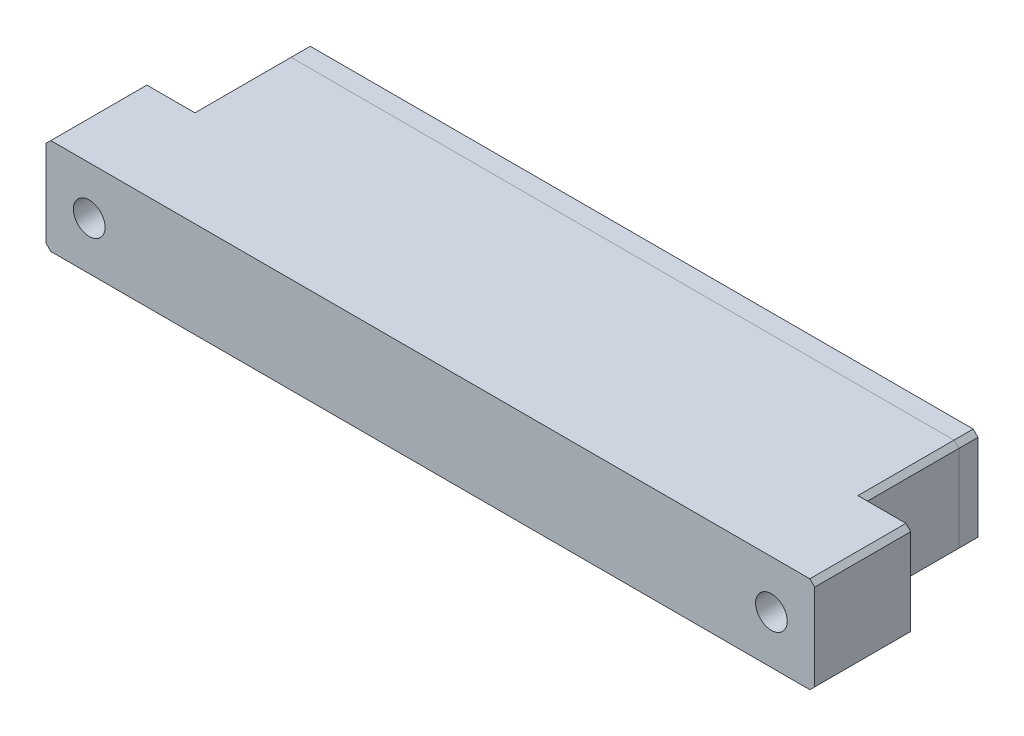
SolidWorks part; units mm, degrees
material "A6063"
ref_plane "Front Plane" through (0, 0, 0) normal (0, 0, 1) x (1, 0, 0)
ref_plane "Top Plane" through (0, 0, 0) normal (0, 1, 0) x (1, 0, 0)
ref_plane "Right Plane" through (0, 0, 0) normal (1, 0, 0) x (0, 0, -1)
sketch "Sketch1" plane through (0, 0, 0) normal (0, 0, 1) x (1, 0, 0)
  line L1 (40, -5) -> (-40, -5)
  line L2 (40, -5) -> (40, 5)
  line L3 (40, 5) -> (-40, 5)
  line L4 (-40, -5) -> (-40, 5)
  line L5 (40, -5) -> (-40, 5) construction
  line L6 (40, 5) -> (-40, -5) construction
  point P0 (0, 0)
  dimension "D1" = 80
  dimension "D2" = 10
extrude "Boss-Extrude1" add sketch "Sketch1" along normal blind 20
sketch "Sketch9" plane through (0, 5, 0) normal (0, 1, 0) x (1, 0, 0)
  line L0 (0, 0) -> (0, -36.7586) construction
  line L1 (40, 0) -> (35, 0)
  line L2 (40, 0) -> (40, -10)
  line L3 (40, -10) -> (35, -10)
  line L4 (35, 0) -> (35, -10)
  line L5 (-40, 0) -> (-35, 0)
  line L6 (-40, 0) -> (-40, -10)
  line L7 (-40, -10) -> (-35, -10)
  line L8 (-35, 0) -> (-35, -10)
  dimension "D1" = 70
  dimension "D2" = 10
extrude "Cut-Extrude3" cut sketch "Sketch9" against normal through all
hole_wizard "M4 Tapped Hole1" positions "Sketch4" profile "Sketch3" tap size "M4" standard "GB"
sketch "Sketch4" plane through (0, 0, 20) normal (0, 0, 1) x (1, 0, 0)
  line L0 (0, 7.9254) -> (0, 0) construction
  line L1 (0, 0) -> (18.9615, 0) construction
  point P0 (-35.5, 0)
  point P1 (35.5, 0)
  dimension "D1" = 71
sketch "Sketch3" plane through (-35.5, 0, 20) normal (1, 0, 0) x (0, -1, 0)
  line L0 (0, 0) -> (0, 8.9914)
  line L1 (0, 8.9914) -> (1.65, 8)
  line L2 (1.65, 8) -> (1.65, 0)
  line L5 (1.65, 0) -> (0, 0)
  line L10 (0, 8.9914) -> (-1.65, 8) construction
  line L11 (0, -6.35) -> (0, 107.95) construction
  dimension "螺纹孔钻头直径" = 3.3
  dimension "螺纹孔钻头深度" = 8
  dimension "导头角度" = 118
cosmetic thread "Cosmetic Thread3" parameters "D1"=8, "D2"=4
cosmetic thread "Cosmetic Thread4" parameters "D1"=8, "D2"=4
hole_wizard "M5 Tapped Hole1" positions "Sketch7" profile "Sketch6" tap size "M5" standard "GB"
sketch "Sketch7" plane through (0, -5, 0) normal (0, -1, 0) x (1, 0, 0)
  line L1 (0, 0) -> (0, 6.5) construction
  line L2 (-35, 0) -> (35, 0) construction
  point P0 (0, 6.5)
  dimension "D1" = 6.5
sketch "Sketch6" plane through (0, -5, 6.5) normal (1, 0, 0) x (0, 0, -1)
  line L0 (0, 0) -> (0, 8)
  line L1 (0, 8) -> (2.1, 8)
  line L2 (2.1, 8) -> (2.1, 0)
  line L5 (2.1, 0) -> (0, 0)
  line L10 (0, 8) -> (-2.1, 8) construction
  line L11 (0, -6.35) -> (0, 107.95) construction
  dimension "螺纹孔钻头直径" = 4.2
  dimension "螺纹孔钻头深度" = 8
  dimension "导头角度" = 180
cosmetic thread "Cosmetic Thread5" parameters "D1"=2, "D2"=5
sketch "Sketch8" plane through (0, 0, 0) normal (0, 0, -1) x (-1, 0, 0)
  line L0 (0, 0) -> (25.8164, 0) construction
  line L2 (-34, 4) -> (34, 4)
  line L3 (-34, 4) -> (-34, -4)
  line L4 (-34, -4) -> (34, -4)
  line L7 (34, 4) -> (34, -4)
  line L8 (0, 0) -> (0, -13.1501) construction
  line L9 (-35, 5) -> (35, 5) construction
  line L10 (35, -5) -> (35, 5) construction
  dimension "D1" = 1
  dimension "D2" = 1
extrude "Cut-Extrude2" cut sketch "Sketch8" against normal blind 3
sketch "Sketch10" plane through (0, 0, 3) normal (0, 0, -1) x (-1, 0, 0)
  line L0 (0, 0) -> (18.7293, 0) construction
  line L1 (-32, 3) -> (32, 3)
  line L2 (-32, 3) -> (-32, -3)
  line L3 (-32, -3) -> (32, -3)
  line L4 (32, 3) -> (32, -3)
  line L5 (0, 0) -> (0, 14.5079) construction
  line L6 (34, 4) -> (-34, 4) construction
  line L7 (34, -4) -> (34, 4) construction
  dimension "D1" = 1
  dimension "D2" = 2
extrude "Cut-Extrude4" cut sketch "Sketch10" against normal blind 3.5
sketch "Sketch11" plane through (0, 0, 3) normal (0, 0, -1) x (-1, 0, 0)
  line L1 (-34, 4) -> (34, 4)
  line L2 (-34, 4) -> (-34, -4)
  line L3 (-34, -4) -> (34, -4)
  line L4 (34, 4) -> (34, -4)
extrude "Boss-Extrude2" add sketch "Sketch11" along normal blind 3 separate body
sketch "Sketch12" plane through (0, 0, 0) normal (0, 0, -1) x (-1, 0, 0)
  line L1 (-35, 5) -> (35, 5)
  line L2 (-35, 5) -> (-35, -5)
  line L3 (-35, -5) -> (35, -5)
  line L4 (35, 5) -> (35, -5)
extrude "Boss-Extrude3" add sketch "Sketch12" along normal blind 2 separate body
sketch "Sketch13" plane through (0, 0, -2) normal (0, 0, -1) x (-1, 0, 0)
  line L0 (0, 0) -> (42.3757, 0) construction
  line L1 (35, -5) -> (35, 5) construction
  circle A0 centre (31.5, 1.5) radius 0.5
  circle A1 centre (31.5, -1.5) radius 0.5
  dimension "D1" = 3
  dimension "D2" = 1
  dimension "D3" = 3.5
extrude "Cut-Extrude5" cut sketch "Sketch13" against normal blind 5
pattern_linear "LPattern1" count 22 spacing 3 along (1, 0, 0) of "Cut-Extrude5"
chamfer "Chamfer1" distance 0.5 angle 45 12 edges at (-40, -5, 15) (-40, 5, 15) (40, -5, 15) (40, 5, 15) (-35, 5, 5) (-35, -5, 5) (35, 5, 5) (35, -5, 5) (-40, 0, 10) (40, 0, 10) (-35, 0, 0) (35, 0, 0)
chamfer "Chamfer2" distance 0.5 angle 45 4 edges at (-35, 5, -1) (-35, -5, -1) (35, 5, -1) (35, -5, -1)
